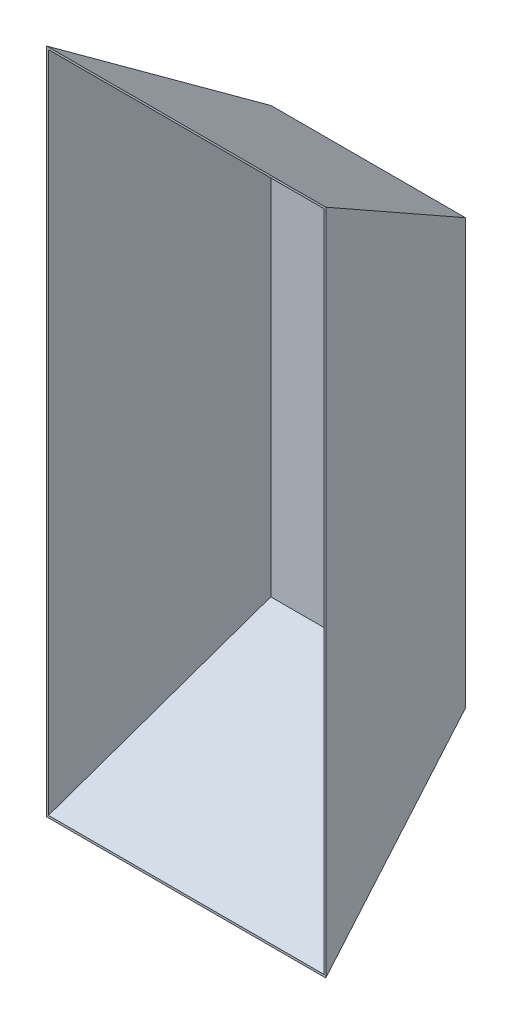
SolidWorks part; units mm, degrees
ref_plane "Front Plane" through (0, 0, 0) normal (0, 0, 1) x (1, 0, 0)
ref_plane "Top Plane" through (0, 0, 0) normal (0, 1, 0) x (1, 0, 0)
ref_plane "Right Plane" through (0, 0, 0) normal (1, 0, 0) x (0, 0, -1)
sketch "Sketch1" plane through (0, 0, 0) normal (0, 0, 1) x (1, 0, 0)
  line L1 (-230, 550) -> (230, 550)
  line L2 (-230, 550) -> (-230, -550)
  line L3 (-230, -550) -> (230, -550)
  line L4 (230, 550) -> (230, -550)
  line L5 (-230, 550) -> (230, -550) construction
  line L6 (-230, -550) -> (230, 550) construction
  point P0 (0, 0)
  dimension "D1" = 1100
  dimension "D2" = 460
extrude "Boss-Extrude1" add sketch "Sketch1" against normal blind 300
sketch "Sketch3" plane through (230, 0, 0) normal (1, 0, 0) x (0, 0, -1)
  line L0 (0, 550) -> (300, 350)
  line L1 (300, -550) -> (300, 550) construction
  line L2 (300, 350) -> (300, 550)
  line L3 (300, 550) -> (0, 550)
  line L4 (0, 0) -> (300, 0) construction
  line L5 (300, -550) -> (0, -550)
  line L6 (300, -350) -> (300, -550)
  line L7 (0, -550) -> (300, -350)
  dimension "D1" = 700
extrude "Cut-Extrude1" cut sketch "Sketch3" against normal through all
sketch "Sketch6" plane through (0, 0, 0) normal (0, 1, 0) x (1, 0, 0)
  line L0 (-230, 0) -> (-160, 300)
  line L1 (-230, 300) -> (230, 300) construction
  line L2 (-160, 300) -> (-230, 300)
  line L3 (-230, 300) -> (-230, 0)
  line L4 (0, 0) -> (0, 202.4784) construction
  line L5 (230, 300) -> (230, 0)
  line L6 (160, 300) -> (230, 300)
  line L7 (230, 0) -> (160, 300)
  dimension "D1" = 320
extrude "Cut-Extrude3" cut sketch "Sketch6" against normal mid plane 1898
shell "Shell1" thickness 3
